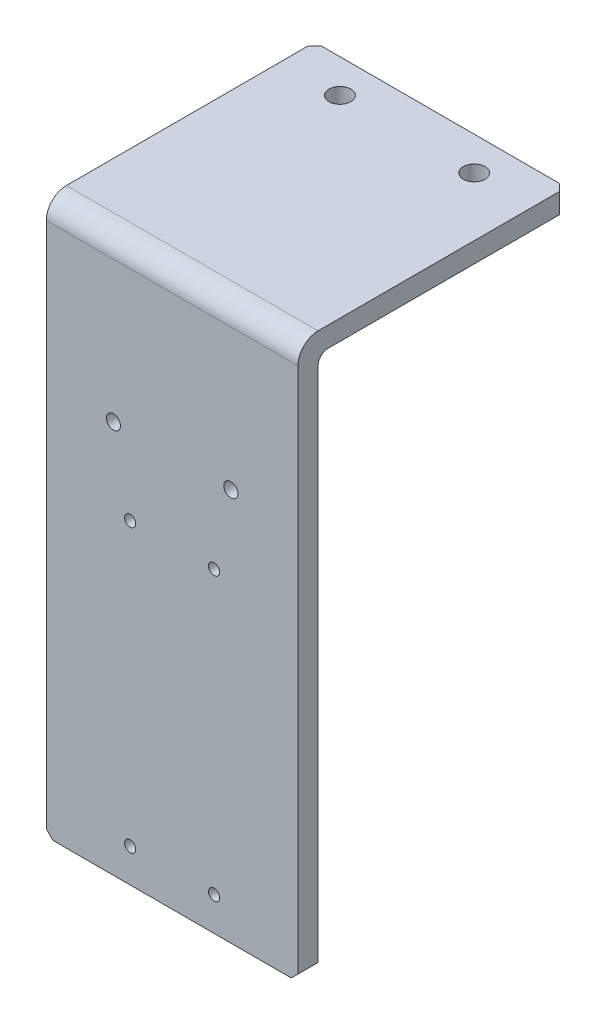
from build123d import *

# Parameters (mm, degrees)
SKETCH1_W                      = 75
SKETCH1_H                      = 165
BOSS_EXTRUDE1_DEPTH            = 80
SHELL1_T                       = -6
FILLET1_R                      = 6
FILLET2_R                      = 3
CHAMFER1_SIZE                  = 2
M4_TAPPED_HOLE1_D              = 3.3
F_6_5_6_5_DIAMETER_HOLE1_D     = 6.5
F_6_5_6_5_DIAMETER_HOLE1_DEPTH = 10
F_6_5_6_5_DIAMETER_HOLE1_TIP   = 1.952797012
M5_TAPPED_HOLE1_D              = 4.2


with BuildPart() as part:
    # Sketch1 → Boss-Extrude1 (new body)
    with BuildSketch(Plane.XY):
        Rectangle(SKETCH1_W, SKETCH1_H)
    extrude(amount=BOSS_EXTRUDE1_DEPTH)

    # Shell1
    shell1_openings = [part.faces().sort_by_distance(p)[0] for p in [
        (0, 0, 0),
        (0, -82.5, 40),
        (-37.5, 0, 40),
        (37.5, 0, 40),
    ]]
    offset(amount=SHELL1_T, openings=shell1_openings, kind=Kind.INTERSECTION)

    # Fillet1
    fillet1_edges = [part.edges().sort_by_distance(p)[0] for p in [
        (0, 82.5, 80),
    ]]
    fillet(fillet1_edges, radius=FILLET1_R)

    # Fillet2
    fillet2_edges = [part.edges().sort_by_distance(p)[0] for p in [
        (0, 76.5, 74),
    ]]
    fillet(fillet2_edges, radius=FILLET2_R)

    # Chamfer1
    chamfer1_edges = [part.edges().sort_by_distance(p)[0] for p in [
        (-37.5, 79.5, 0),
        (37.5, 79.5, 0),
        (37.5, -82.5, 77),
        (-37.5, -82.5, 77),
    ]]
    chamfer(chamfer1_edges, length=CHAMFER1_SIZE)

    # M4 Tapped Hole1 (through all)
    with Locations(Plane(origin=(0, 0, 74), x_dir=(-1, 0, 0), z_dir=(0, 0, -1))):
        with Locations((-12.5, -72.5), (-12.5, 11.5), (12.5, 11.5), (12.5, -72.5)):
            Hole(M4_TAPPED_HOLE1_D / 2)

    # Ø6.5 (6.5) Diameter Hole1
    with Locations(Plane.XZ.offset(-76.5)):
        with Locations((-20, 10), (20, 10)):
            Hole(F_6_5_6_5_DIAMETER_HOLE1_D / 2, depth=F_6_5_6_5_DIAMETER_HOLE1_DEPTH)
            with Locations((0, 0, -(F_6_5_6_5_DIAMETER_HOLE1_DEPTH + F_6_5_6_5_DIAMETER_HOLE1_TIP / 2))):  # 118° drill point
                Cone(0, F_6_5_6_5_DIAMETER_HOLE1_D / 2, F_6_5_6_5_DIAMETER_HOLE1_TIP, mode=Mode.SUBTRACT)

    # M5 Tapped Hole1 (through all)
    with Locations(Plane(origin=(0, 0, 74), x_dir=(-1, 0, 0), z_dir=(0, 0, -1))):
        with Locations((-17.5, 34.5), (17.5, 34.5)):
            Hole(M5_TAPPED_HOLE1_D / 2)


solid = part.part
